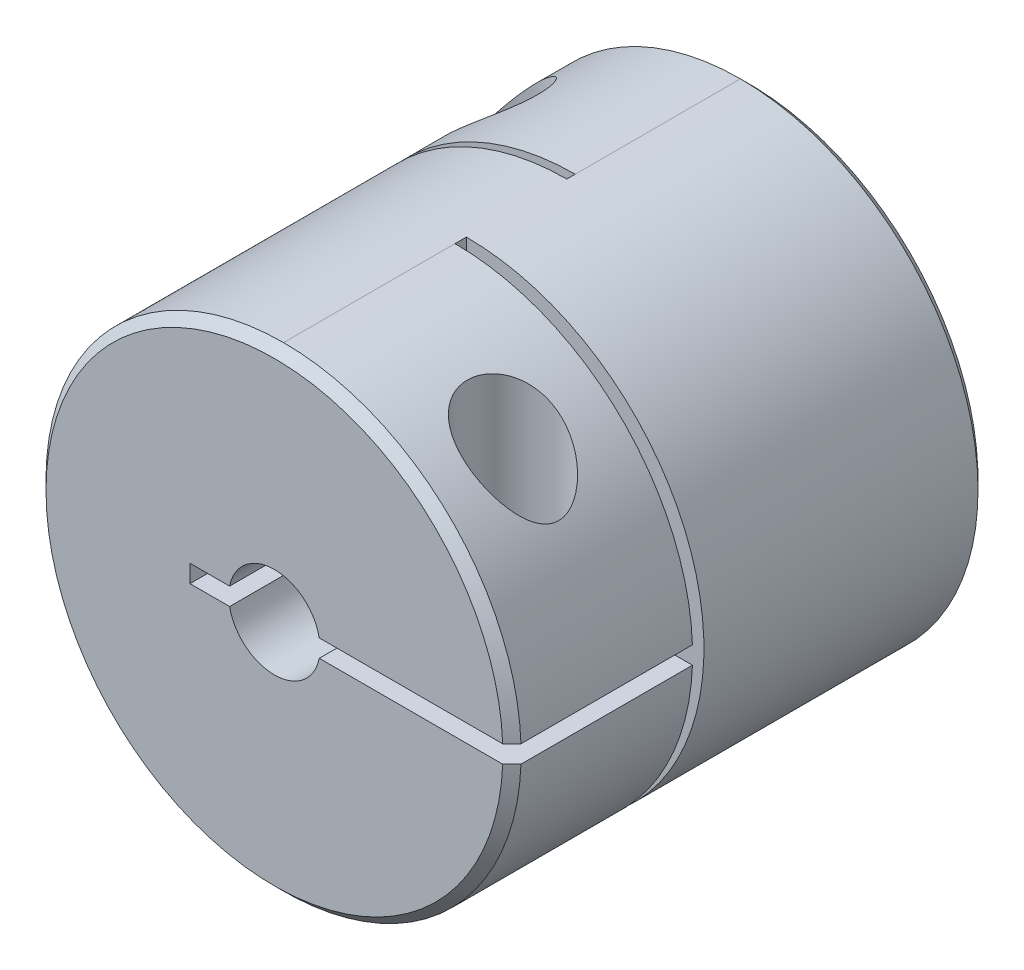
from build123d import *

# Parameters (mm, degrees)
SKETCH_1_R          = 13
EXTRUDE_1_DEPTH     = 26
SKETCH_2_R          = 2.5
CUT_EXTRUDE_1_DEPTH = 32.843366656
SKETCH_3_R          = 5
CUT_EXTRUDE_2_DEPTH = 12
SKETCH_4_W          = 21.947389444
SKETCH_4_H          = 0.965950114
CUT_EXTRUDE_3_DEPTH = 10
SKETCH_5_W          = 24.42165542
SKETCH_5_H          = 0.576488958
CUT_EXTRUDE_4_DEPTH = 10
SKETCH_6_W          = 0.620030038
SKETCH_6_H          = 28.40124723
CUT_EXTRUDE_5_DEPTH = 32.843366656
SKETCH_7_W          = 0.460474017
SKETCH_7_H          = 28.978503402
CUT_EXTRUDE_6_DEPTH = 32.843366656
CHAMFER_1_SIZE      = 0.5


with BuildPart() as part:
    # 草图1 → 凸台-拉伸1 (new body)
    with BuildSketch(Plane.XY):
        with Locations(Location((0, 0, 0), (0, 0, 180))):
            Circle(SKETCH_1_R)
    extrude(amount=EXTRUDE_1_DEPTH)

    # 草图2 → 切除-拉伸1 (cut, through all)
    with BuildSketch(Plane.XY.offset(26)):
        Circle(SKETCH_2_R)
    extrude(amount=-CUT_EXTRUDE_1_DEPTH, mode=Mode.SUBTRACT)

    # 草图3 → 切除-拉伸2 (cut)
    with BuildSketch(Plane(origin=(0, 0, 0), x_dir=(-1, 0, 0), z_dir=(0, 0, -1))):
        Circle(SKETCH_3_R)
    extrude(amount=-CUT_EXTRUDE_2_DEPTH, mode=Mode.SUBTRACT)

    # 草图4 → 切除-拉伸3 (cut)
    with BuildSketch(Plane.XY.offset(26)):
        with Locations((6.353035437, 0)):
            Rectangle(SKETCH_4_W, SKETCH_4_H)
    extrude(amount=-CUT_EXTRUDE_3_DEPTH, mode=Mode.SUBTRACT)

    # 草图5 → 切除-拉伸4 (cut)
    with BuildSketch(Plane(origin=(0, 0, 0), x_dir=(-1, 0, 0), z_dir=(0, 0, -1))):
        with Locations((6.383187544, 0)):
            Rectangle(SKETCH_5_W, SKETCH_5_H)
    extrude(amount=-CUT_EXTRUDE_4_DEPTH, mode=Mode.SUBTRACT)

    # 草图6 → 切除-拉伸5 (cut, through all)
    with BuildSketch(Plane(origin=(0, 0, 0), x_dir=(0, 0, -1), z_dir=(1, 0, 0))):
        with Locations((-15.807983144, 0.215959177)):
            Rectangle(SKETCH_6_W, SKETCH_6_H)
    extrude(amount=CUT_EXTRUDE_5_DEPTH, mode=Mode.SUBTRACT)

    # 草图7 → 切除-拉伸6 (cut, through all)
    with BuildSketch(Plane(origin=(0, 0, 0), x_dir=(0, 0, -1), z_dir=(1, 0, 0))):
        with Locations((-9.770664876, -0.784834467)):
            Rectangle(SKETCH_7_W, SKETCH_7_H)
    extrude(amount=-CUT_EXTRUDE_6_DEPTH, mode=Mode.SUBTRACT)

    # 草图8 → 切除-旋转1 (revolve, cut)
    with BuildSketch(Plane.XY.offset(21), mode=Mode.PRIVATE) as cut_revolve_1_sk:
        Polygon((5.554054174, 13), (5.554054174, 3.477242408), (6.804054174, 3.477242408), (6.804054174, -12.992472662), (8.054054174, -12.992472662), (8.054054174, 13), align=None)
    revolve(cut_revolve_1_sk.sketch.rotate(Axis((8.054054174, 16.145548825, 21), (0, -1, 0)), 270), axis=Axis((8.054054174, 16.145548825, 21), (0, -1, 0)), mode=Mode.SUBTRACT)

    # 草图9 → 切除-旋转2 (revolve, cut)
    with BuildSketch(Plane(origin=(0, 0, 5), x_dir=(-1, 0, 0), z_dir=(0, 0, -1)), mode=Mode.PRIVATE) as cut_revolve_2_sk:
        Polygon((6.601636039, 12.445267502), (6.601636039, 3.589776819), (7.851636039, 3.589776819), (7.851636039, -11.887089541), (9.101636039, -11.887089541), (9.101636039, 12.445267502), align=None)
    revolve(cut_revolve_2_sk.sketch.rotate(Axis((-9.101636039, 15.747906526, 5), (0, -1, 0)), 180), axis=Axis((-9.101636039, 15.747906526, 5), (0, -1, 0)), mode=Mode.SUBTRACT)

    # 倒角1
    chamfer_1_edges = [part.edges().sort_by_distance(p)[0] for p in [
        (-0.241529218, 12.9977561, 26),
        (13, 0, 0),
    ]]
    chamfer(chamfer_1_edges, length=CHAMFER_1_SIZE)


solid = part.part
